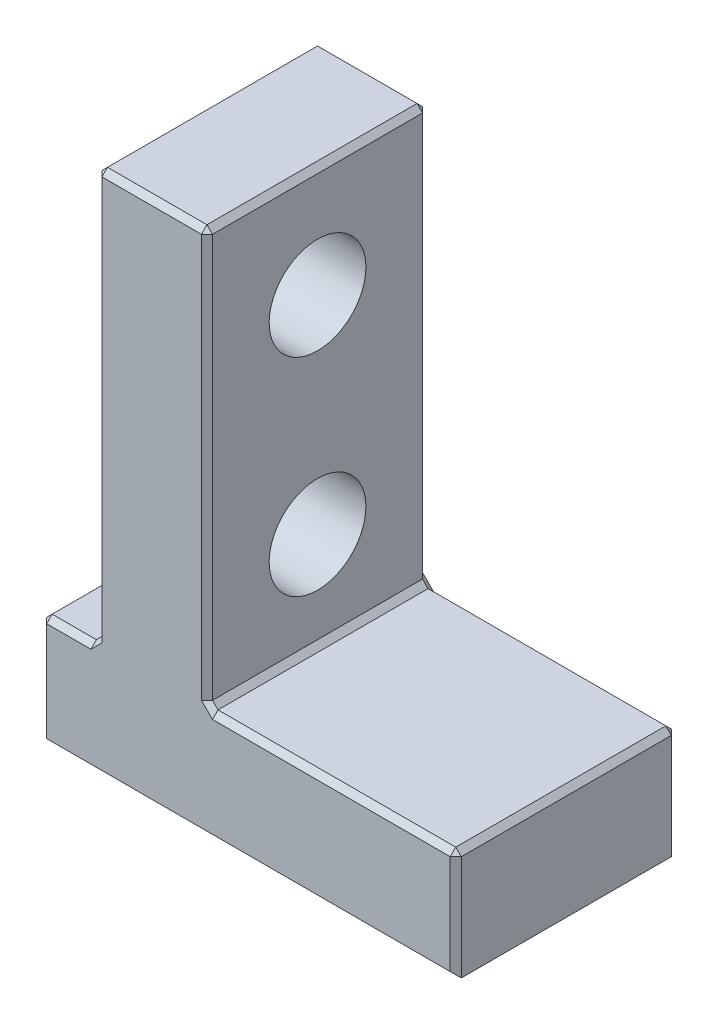
SolidWorks part; units mm, degrees
ref_plane "Front Plane" through (0, 0, 0) normal (0, 0, 1) x (1, 0, 0)
ref_plane "Top Plane" through (0, 0, 0) normal (0, 1, 0) x (1, 0, 0)
ref_plane "Right Plane" through (0, 0, 0) normal (1, 0, 0) x (0, 0, -1)
sketch "Sketch2" plane through (0, 0, 0) normal (0, 0, 1) x (1, 0, 0)
  line L0 (-10.794, 0) -> (-8.794, 0)
  line L1 (-8.794, 0) -> (-8.794, 15)
  line L2 (-8.794, 15) -> (-4.794, 15)
  line L3 (-4.794, 15) -> (-4.794, 0)
  line L4 (-10.794, 0) -> (-10.794, -4)
  line L5 (-10.794, -4) -> (4.206, -4)
  line L6 (4.206, -4) -> (4.206, 0)
  line L7 (-4.794, 0) -> (4.206, 0)
  dimension "D1" = 15
  dimension "D2" = 15
  dimension "D3" = 4
  dimension "D4" = 4
  dimension "D5" = 2
extrude "Boss-Extrude1" add sketch "Sketch2" along normal blind 8
chamfer "Chamfer1" distance 0.2 angle 45 23 edges at (-4.794, 15, 4) (-8.794, 15, 4) (-10.794, -4, 4) (-3.294, -4, 0) (4.206, -2, 0) (-4.794, 7.5, 0) (-6.794, 15, 0) (-8.794, 7.5, 0) (-10.794, -2, 0) (-8.794, 0, 4) (-9.794, 0, 0) (-10.794, 0, 4) (4.206, 0, 4) (-0.294, 0, 0) (-4.794, 0, 4) (-9.794, 0, 8) (-8.794, 7.5, 8) (-6.794, 15, 8) (-4.794, 7.5, 8) (-0.294, 0, 8) (4.206, -2, 8) (-3.294, -4, 8) (-10.794, -2, 8)
sketch "Sketch4" plane through (-8.794, 0, 0) normal (-1, 0, 0) x (0, 0, 1)
  line L0 (4, 17.1628) -> (4, -5.9791) construction
  line L1 (-3.9763, 7.25) -> (15.3304, 7.25) construction
  line L2 (7.8, 0) -> (0.2, 0) construction
  circle A0 centre (4, 11) radius 1.75
  circle A1 centre (4, 3.5) radius 1.75
  dimension "D1" = 3.5
  dimension "D2" = 3.5
  dimension "D3" = 7.5
extrude "Cut-Extrude1" cut sketch "Sketch4" against normal up to next and the other way through all
